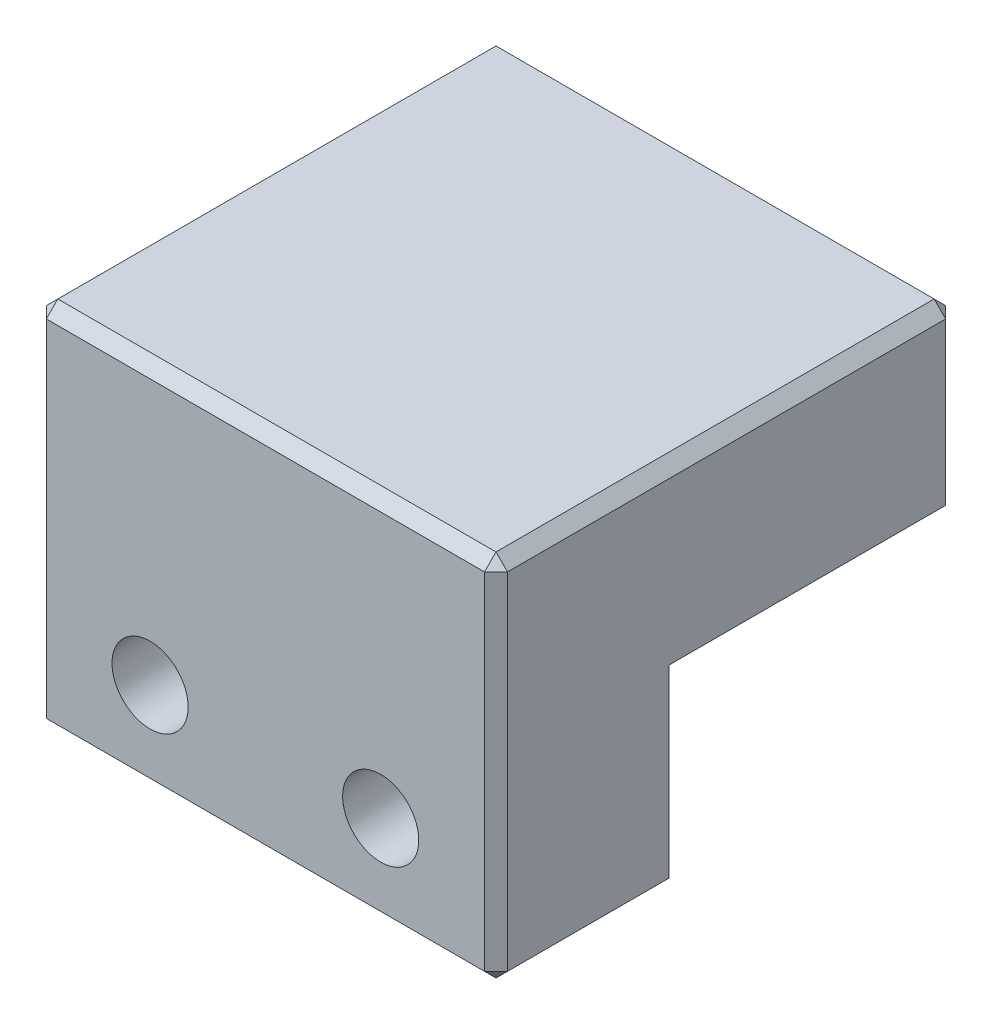
from build123d import *

# Parameters (mm, degrees)
SKETCH_1_W             = 20
SKETCH_1_H             = 20
EXTRUDE_1_DEPTH        = 8
HOLE_WIZARD_M4_1_D     = 3.3
HOLE_WIZARD_M4_1_DEPTH = 14.1
HOLE_WIZARD_M4_1_TIP   = 0.991420021
SKETCH_6_W             = 20
SKETCH_6_H             = 8
EXTRUDE_2_DEPTH        = 8
HOLE_WIZARD_M4_3_D     = 3.3
HOLE_WIZARD_M4_3_DEPTH = 14.1
HOLE_WIZARD_M4_3_TIP   = 0.991420021
CHAMFER_2_SIZE         = 0.5


with BuildPart() as part:
    # 草图1 → 凸台-拉伸1 (new body)
    with BuildSketch(Plane(origin=(0, 0, 0), x_dir=(1, 0, 0), z_dir=(0, 1, 0))):
        Rectangle(SKETCH_1_W, SKETCH_1_H)
    extrude(amount=EXTRUDE_1_DEPTH)

    # M4 螺纹孔1
    with Locations(Plane(origin=(-10, -0.113114855, 4.919036023), x_dir=(0, 0, -1), z_dir=(-1, 0, 0))):
        with Locations((9.919036023, -4.113114855), (-0.080963977, -4.113114855)):
            Hole(HOLE_WIZARD_M4_1_D / 2, depth=HOLE_WIZARD_M4_1_DEPTH)
            with Locations((0, 0, -(HOLE_WIZARD_M4_1_DEPTH + HOLE_WIZARD_M4_1_TIP / 2))):  # 118° drill point
                Cone(0, HOLE_WIZARD_M4_1_D / 2, HOLE_WIZARD_M4_1_TIP, mode=Mode.SUBTRACT)

    # 草图6 → 凸台-拉伸2 (add)
    with BuildSketch(Plane.XY.offset(10)):
        with Locations((0, -4)):
            Rectangle(SKETCH_6_W, SKETCH_6_H)
    extrude(amount=-EXTRUDE_2_DEPTH)

    # M4 螺纹孔3
    with Locations(Plane.XY.offset(10)):
        with Locations((-5, -4), (5, -4)):
            Hole(HOLE_WIZARD_M4_3_D / 2, depth=HOLE_WIZARD_M4_3_DEPTH)
            with Locations((0, 0, -(HOLE_WIZARD_M4_3_DEPTH + HOLE_WIZARD_M4_3_TIP / 2))):  # 118° drill point
                Cone(0, HOLE_WIZARD_M4_3_D / 2, HOLE_WIZARD_M4_3_TIP, mode=Mode.SUBTRACT)

    # 倒角2
    chamfer_2_edges = [part.edges().sort_by_distance(p)[0] for p in [
        (-10, 8, 0),
        (-10, 0, 10),
        (-10, -4, 2),
        (-10, 0, -4),
        (10, 4, -10),
        (0, 8, -10),
        (-10, 4, -10),
        (0, 0, -10),
        (10, -8, 6),
        (10, 0, -4),
        (10, -4, 2),
        (0, -8, 2),
        (-10, -8, 6),
        (0, -8, 10),
        (10, 8, 0),
        (0, 8, 10),
        (10, 0, 10),
        (-10, 4, 3.35),
        (-10, 4, -6.65),
    ]]
    chamfer(chamfer_2_edges, length=CHAMFER_2_SIZE)


solid = part.part
